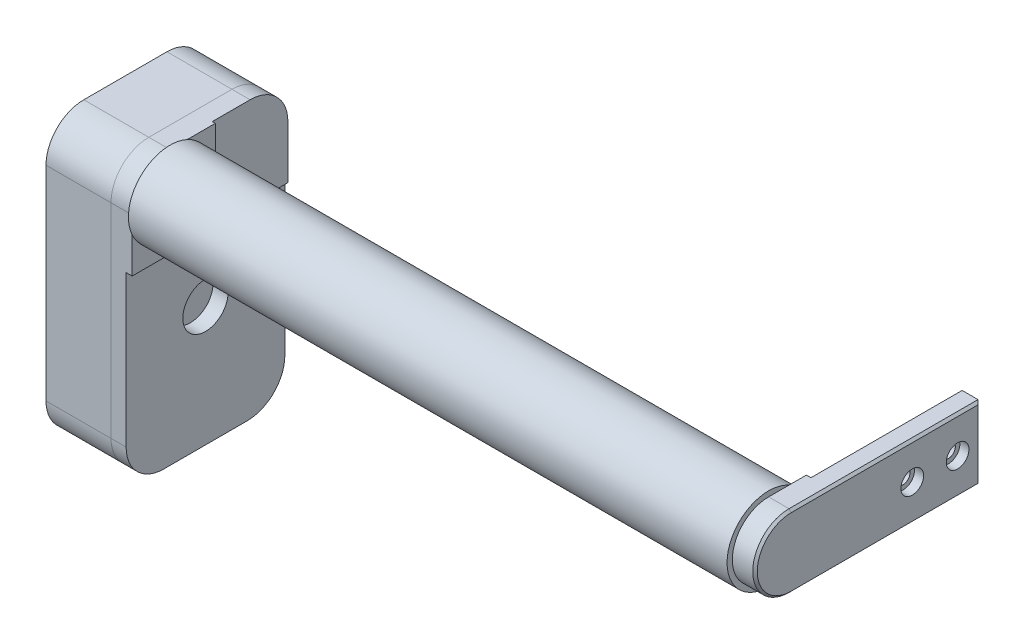
from build123d import *

# Parameters (mm, degrees)
EXTRUDE_1_DEPTH           = 15
SKETCH_2_R                = 27.5
EXTRUDE_2_DEPTH           = 396
HOLE_WIZARD_1_D           = 9
HOLE_WIZARD_1_CBORE_D     = 15
HOLE_WIZARD_1_CBORE_DEPTH = 6
CHAMFER_1_SIZE            = 1.5
SKETCH_5_W                = 3
SKETCH_5_H                = 100
CUT_EXTRUDE_1_DEPTH       = 410.351010748
SKETCH_6_R                = 8
EXTRUDE_3_DEPTH           = 25
EXTRUDE_4_DEPTH           = 14
SKETCH_8_W                = 4
SKETCH_8_H                = 125
CUT_EXTRUDE_2_DEPTH       = 464.030506554
SKETCH_9_R                = 15
CUT_EXTRUDE_3_DEPTH       = 454.789598823
SKETCH_10_W               = 2
SKETCH_10_H               = 50
CUT_EXTRUDE_4_DEPTH       = 469.578702034
EXTRUDE_5_DEPTH           = 43


with BuildPart() as part:
    # 草图1 → 凸台-拉伸1 (new body)
    with BuildSketch(Plane(origin=(0, 0, 0), x_dir=(0, 0, -1), z_dir=(1, 0, 0))):
        with BuildLine():
            Line((-62.5, 24), (62.5, 24))
            Line((62.5, 24), (62.5, -24))
            Line((62.5, -24), (-62.5, -24))
            ThreePointArc((-62.5, -24), (-86.5, 0), (-62.5, 24))
        make_face()
    extrude(amount=EXTRUDE_1_DEPTH)

    # 草图2 → 凸台-拉伸2 (add)
    with BuildSketch(Plane.ZY):
        with Locations(Location((62.5, 0, 0), (0, 0, 240.777129706))):
            Circle(SKETCH_2_R)
    extrude(amount=EXTRUDE_2_DEPTH)

    # 打孔尺寸(%根据)内六角花形圆柱头螺钉1 (through all)
    with Locations(Plane(origin=(15, 0, 0), x_dir=(0, 0, -1), z_dir=(1, 0, 0))):
        with Locations((17.5, 0), (47.5, 0)):
            CounterBoreHole(HOLE_WIZARD_1_D / 2, HOLE_WIZARD_1_CBORE_D / 2, HOLE_WIZARD_1_CBORE_DEPTH)

    # 倒角1
    chamfer_1_edges = [part.edges().sort_by_distance(p)[0] for p in [
        (15, 0, 86.5),
        (15, -24, 0),
        (15, 0, -62.5),
        (15, 24, 0),
    ]]
    chamfer(chamfer_1_edges, length=CHAMFER_1_SIZE)

    # 草图5 → 切除-拉伸1 (cut, through all)
    with BuildSketch(Plane(origin=(0, 24, 0), x_dir=(1, 0, 0), z_dir=(0, 1, 0))):
        with Locations((1.5, 12.5)):
            Rectangle(SKETCH_5_W, SKETCH_5_H)
    extrude(amount=-CUT_EXTRUDE_1_DEPTH, mode=Mode.SUBTRACT)

    # 草图6 → 凸台-拉伸3 (add)
    with BuildSketch(Plane.ZY.offset(396)):
        with Locations((62.5, 0)):
            Circle(SKETCH_6_R)
    extrude(amount=EXTRUDE_3_DEPTH)

    # 草图7 → 凸台-拉伸4 (add)
    with BuildSketch(Plane.ZY.offset(396)):
        with BuildLine():
            Line((7.5, 25), (62.5, 25))
            ThreePointArc((62.5, 25), (80.17766953, 17.67766953), (87.5, 0))
            Line((87.5, 0), (87.5, -135))
            ThreePointArc((87.5, -135), (80.17766953, -152.67766953), (62.5, -160))
            Line((62.5, -160), (7.5, -160))
            ThreePointArc((7.5, -160), (-10.17766953, -152.67766953), (-17.5, -135))
            Line((-17.5, -135), (-17.5, 0))
            ThreePointArc((-17.5, 0), (-10.17766953, 17.67766953), (7.5, 25))
        make_face()
    extrude(amount=EXTRUDE_4_DEPTH)

    # 草图8 → 切除-拉伸2 (cut, through all)
    with BuildSketch(Plane(origin=(0, 0, -17.5), x_dir=(-1, 0, 0), z_dir=(0, 0, -1))):
        with Locations((398, -97.5)):
            Rectangle(SKETCH_8_W, SKETCH_8_H)
    extrude(amount=-CUT_EXTRUDE_2_DEPTH, mode=Mode.SUBTRACT)

    # 草图9 → 切除-拉伸3 (cut, through all)
    with BuildSketch(Plane(origin=(-400, 0, 0), x_dir=(0, 0, -1), z_dir=(1, 0, 0))):
        with Locations((-35, -80)):
            Circle(SKETCH_9_R)
    extrude(amount=-CUT_EXTRUDE_3_DEPTH, mode=Mode.SUBTRACT)

    # 草图10 → 切除-拉伸4 (cut, through all)
    with BuildSketch(Plane(origin=(0, 25, 0), x_dir=(1, 0, 0), z_dir=(0, 1, 0))):
        with Locations((-397, -7.5)):
            Rectangle(SKETCH_10_W, SKETCH_10_H)
    extrude(amount=-CUT_EXTRUDE_4_DEPTH, mode=Mode.SUBTRACT)


with BuildPart() as body_2:
    # 草图11 → 凸台-拉伸5 (new body)
    with BuildSketch(Plane.ZY.offset(410)):
        with BuildLine():
            Line((62.5, 25), (7.5, 25))
            ThreePointArc((7.5, 25), (-10.17766953, 17.67766953), (-17.5, 0))
            Line((-17.5, 0), (-17.5, -135))
            ThreePointArc((-17.5, -135), (-10.17766953, -152.67766953), (7.5, -160))
            Line((7.5, -160), (62.5, -160))
            ThreePointArc((62.5, -160), (80.17766953, -152.67766953), (87.5, -135))
            Line((87.5, -135), (87.5, 0))
            ThreePointArc((87.5, 0), (80.17766953, 17.67766953), (62.5, 25))
        make_face()
    extrude(amount=EXTRUDE_5_DEPTH)


solid = Compound([part.part, body_2.part])
